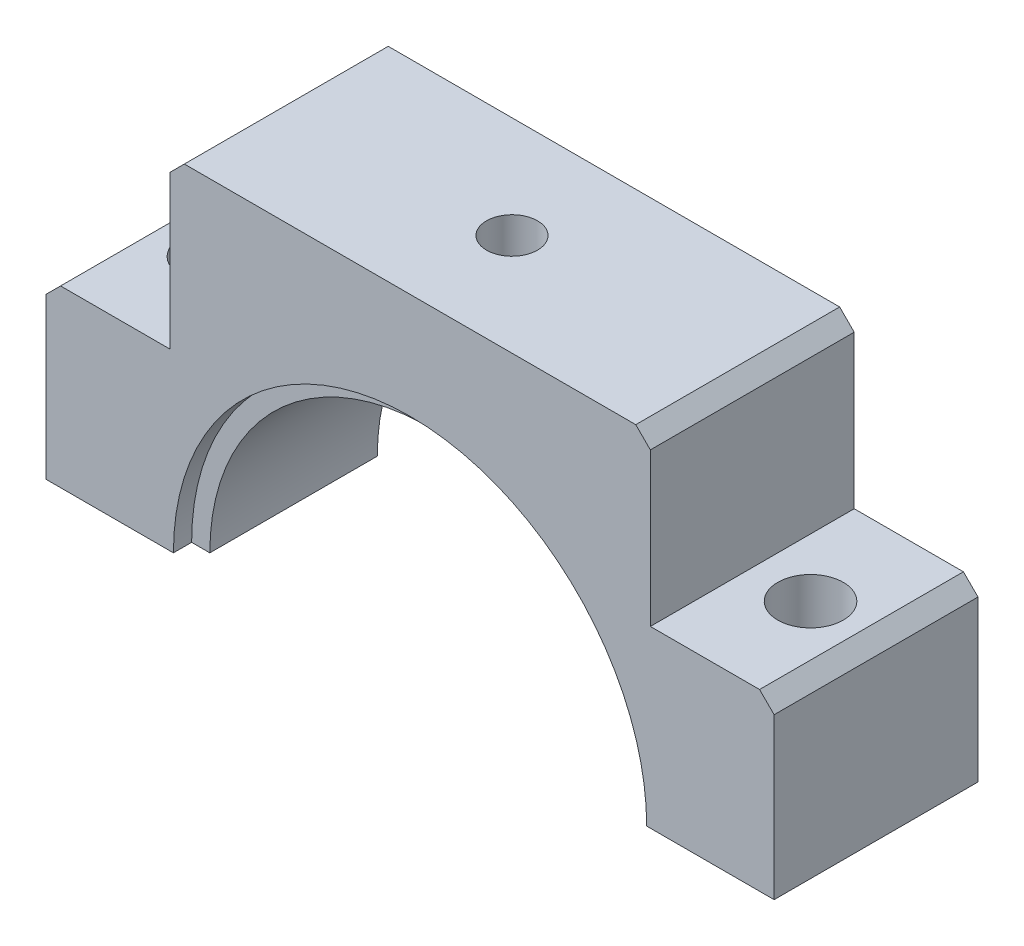
SolidWorks part; units mm, degrees
material "Q235-A"
ref_plane "Front Plane" through (0, 0, 0) normal (0, 0, 1) x (1, 0, 0)
ref_plane "Top Plane" through (0, 0, 0) normal (0, 1, 0) x (1, 0, 0)
ref_plane "Right Plane" through (0, 0, 0) normal (1, 0, 0) x (0, 0, -1)
sketch "Sketch1" plane through (0, 0, 0) normal (0, 0, 1) x (1, 0, 0)
  line L0 (-50, 24) -> (-33, 24)
  line L1 (-50, 0) -> (-30, 0)
  line L2 (-50, 0) -> (-50, 24)
  line L3 (-33, 47) -> (33, 47)
  line L5 (-33, 24) -> (-33, 47)
  line L6 (0, 58.7143) -> (0, -17.0907) construction
  line L7 (50, 0) -> (50, 24)
  line L8 (50, 24) -> (33, 24)
  line L9 (33, 24) -> (33, 47)
  line L10 (30, 0) -> (50, 0)
  arc A0 (30, 0) -> (-30, 0) centre (0, 0) ccw
  point P13 (0, 47)
  dimension "D1" = 100
  dimension "D2" = 47
  dimension "D3" = 23
  dimension "D4" = 33
extrude "Boss-Extrude1" add sketch "Sketch1" along normal blind 28
chamfer "Chamfer1" distance 2 angle 45 4 edges at (50, 24, 14) (33, 47, 14) (-33, 47, 14) (-50, 24, 14)
sketch "Sketch2" plane through (0, 47, 0) normal (0, 1, 0) x (1, 0, 0)
  line L0 (50, -14) -> (-50, -14)
  line L2 (50, 0) -> (50, -28) construction
  line L3 (-50, -28) -> (-50, 0) construction
  line L4 (-41, -9.0808) -> (-41, -18.9192)
  line L5 (41, -9.0808) -> (41, -18.9192)
  point P10 (-41, -14)
  point P11 (41, -14)
  dimension "D1" = 100
  dimension "D2" = 82
  dimension "D3" = 9
hole_wizard "M8x1.0 Tapped Hole1" positions "Sketch3" profile "Sketch4" tap size "M8x1.0" standard "GB"
sketch "Sketch3" plane through (0, 47, 0) normal (0, 1, 0) x (1, 0, 0)
  line L0 (50, -14) -> (-50, -14) construction
  point P0 (0, -14)
sketch "Sketch4" plane through (0, 47, 14) normal (1, 0, 0) x (0, 0, 1)
  line L0 (0, 0) -> (0, 15.103)
  line L1 (0, 15.103) -> (3.5, 13)
  line L2 (3.5, 13) -> (3.5, 0)
  line L5 (3.5, 0) -> (0, 0)
  line L10 (0, 15.103) -> (-3.5, 13) construction
  line L11 (0, -6.35) -> (0, 107.95) construction
  dimension "螺纹孔钻头直径" = 7
  dimension "螺纹孔钻头深度" = 13
  dimension "导头角度" = 118
cosmetic thread "Cosmetic Thread1" parameters "D1"=8, "D2"=8
hole_wizard "Hole2" positions "Sketch9" profile "Sketch10" legacy end condition through all
sketch "Sketch9" plane through (0, 24, 0) normal (0, 1, 0) x (1, 0, 0)
  line L0 (-41, -9.0808) -> (-41, -18.9192) construction
  line L1 (41, -9.0808) -> (41, -18.9192) construction
  point P0 (-41, -14)
  point P4 (41, -14)
sketch "Sketch10" plane through (-41, 24, 14) normal (1, 0, 0) x (0, 0, 1)
  line L0 (0, 0) -> (0, 24)
  line L1 (0, 24) -> (4.5, 24)
  line L2 (4.5, 24) -> (4.5, 0)
  line L3 (4.5, 0) -> (0, 0)
  line L4 (0, 110) -> (0, -10) construction
  dimension "直径" = 9
  dimension "深度" = 24
sketch "Sketch15" plane through (0, 0, 0) normal (0, 0, -1) x (-1, 0, 0)
  circle A0 centre (0, 0) radius 32.5
extrude "Cut-Extrude3" cut sketch "Sketch15" against normal blind 2.5
sketch "Sketch16" plane through (0, 0, 28) normal (0, 0, 1) x (1, 0, 0)
  circle A1 centre (0, 0) radius 32.5
  circle A2 centre (0, 0) radius 32.5
  dimension "D1" = 0
extrude "Cut-Extrude4" cut sketch "Sketch16" against normal blind 2.5
hole_wizard "Hole3" positions "Sketch18" profile "Sketch19" legacy end condition through all
sketch "Sketch18" plane through (0, 47, 0) normal (0, 1, 0) x (1, 0, 0)
  point P0 (0, -14)
sketch "Sketch19" plane through (0, 47, 14) normal (1, 0, 0) x (0, 0, 1)
  line L0 (0, 0) -> (0, 47)
  line L1 (0, 47) -> (2, 47)
  line L2 (2, 47) -> (2, 0)
  line L3 (2, 0) -> (0, 0)
  line L4 (0, 110) -> (0, -10) construction
  dimension "直径" = 4
  dimension "深度" = 47
